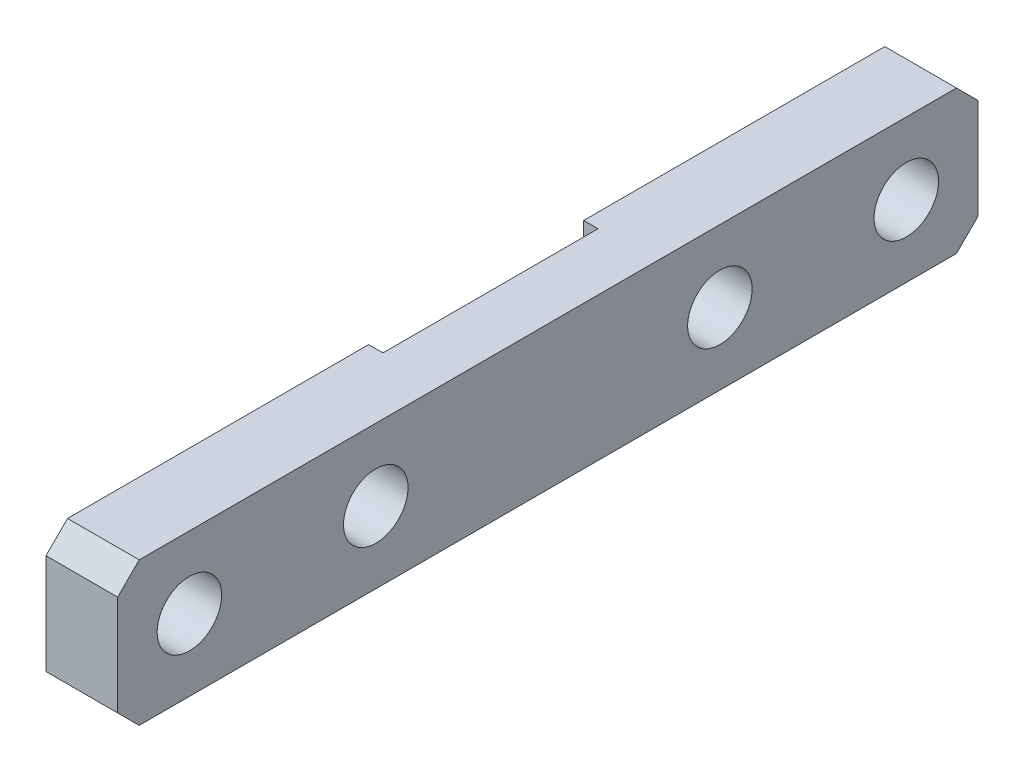
SolidWorks part; units mm, degrees
ref_plane "前视基准面" through (0, 0, 0) normal (0, 0, 1) x (1, 0, 0)
ref_plane "上视基准面" through (0, 0, 0) normal (0, 1, 0) x (1, 0, 0)
ref_plane "右视基准面" through (0, 0, 0) normal (1, 0, 0) x (0, 0, -1)
sketch "草图1" plane through (0, 0, 0) normal (1, 0, 0) x (0, 0, -1)
  line L1 (-60, 10) -> (60, 10)
  line L2 (-60, 10) -> (-60, -10)
  line L3 (-60, -10) -> (60, -10)
  line L4 (60, 10) -> (60, -10)
  line L5 (-60, 10) -> (60, -10) construction
  line L6 (-60, -10) -> (60, 10) construction
  point P0 (0, 0)
  dimension "D1" = 120
  dimension "D2" = 20
extrude "凸台-拉伸1" add sketch "草图1" along normal blind 10
hole_wizard "Ø9.0 (9) 直径孔1" positions "草图2" profile "草图3" hole size "Ø9.0" standard "GB" end condition through all
sketch "草图2" plane through (10, 0, 0) normal (1, 0, 0) x (0, 0, -1)
  line L0 (0, 0) -> (0, 19.1379) construction
  point P0 (-24, 0)
  point P2 (24, 0)
  dimension "D1" = 48
sketch "草图3" plane through (10, 0, 24) normal (0, 1, 0) x (0, 0, -1)
  line L0 (0, 0) -> (0, 10)
  line L1 (0, 10) -> (4.5, 10)
  line L2 (4.5, 10) -> (4.5, 0)
  line L5 (4.5, 0) -> (0, 0)
  line L11 (0, -6.35) -> (0, 107.95) construction
  dimension "通孔孔直径" = 9
  dimension "通孔孔深度" = 10
hole_wizard "Ø9.0 (9) 直径孔2" positions "草图4" profile "草图5" hole size "Ø9.0" standard "GB" end condition through all
sketch "草图4" plane through (0, 0, 0) normal (-1, 0, 0) x (0, 0, 1)
  line L0 (0, 0) -> (0, 29.4039) construction
  point P0 (-50, 0)
  point P2 (50, 0)
  dimension "D1" = 100
sketch "草图5" plane through (0, 0, -50) normal (0, 1, 0) x (0, 0, 1)
  line L0 (0, 0) -> (0, 10)
  line L1 (0, 10) -> (4.5, 10)
  line L2 (4.5, 10) -> (4.5, 0)
  line L5 (4.5, 0) -> (0, 0)
  line L11 (0, -6.35) -> (0, 107.95) construction
  dimension "通孔孔直径" = 9
  dimension "通孔孔深度" = 10
sketch "草图6" plane through (0, 0, 0) normal (1, 0, 0) x (0, 0, -1)
  line L0 (-60, -10) -> (60, -10) construction
  line L5 (-15, 10) -> (15, 10)
  line L6 (-15, 10) -> (-15, -10)
  line L7 (-15, -10) -> (15, -10)
  line L8 (15, 10) -> (15, -10)
  line L9 (-15, 10) -> (15, -10) construction
  line L10 (-15, -10) -> (15, 10) construction
  point P0 (0, 0)
  dimension "D1" = 30
extrude "切除-拉伸1" cut sketch "草图6" along normal blind 2
chamfer "倒角1" distance 3 angle 45 4 edges at (5, -10, -60) (5, 10, -60) (5, -10, 60) (5, 10, 60)
